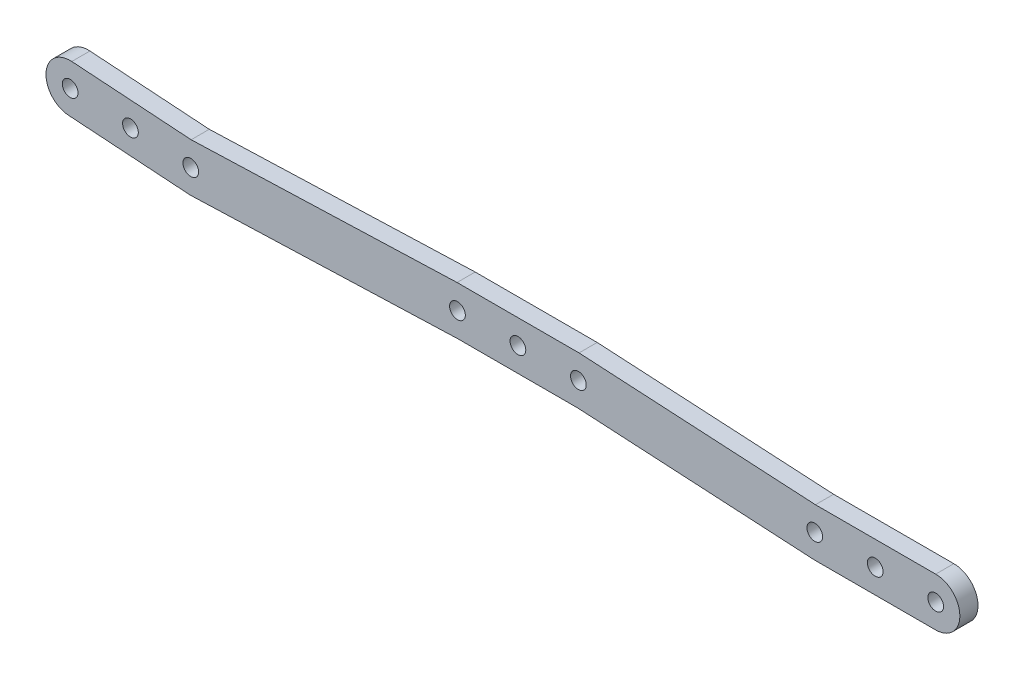
SolidWorks part; units mm, degrees
ref_plane "Front Plane" through (0, 0, 0) normal (0, 0, 1) x (1, 0, 0)
ref_plane "Top Plane" through (0, 0, 0) normal (0, 1, 0) x (1, 0, 0)
ref_plane "Right Plane" through (0, 0, 0) normal (1, 0, 0) x (0, 0, -1)
other "Configuration Table"
sketch "Sketch3" plane through (0, 0, 0) normal (0, 0, 1) x (1, 0, 0)
  line L8 (52.491, -11.9324) -> (42.491, -11.9324) construction
  line L9 (42.491, -11.9324) -> (32.491, -11.9324) construction
  line L10 (32.491, -11.9324) -> (-6.6156, -9.7382) construction
  line L11 (-6.6156, -9.7382) -> (-16.6156, -9.7382) construction
  line L12 (-16.6156, -9.7382) -> (-26.6156, -9.7382) construction
  line L13 (-26.6156, -9.7382) -> (-70.7349, -11.2865) construction
  line L14 (-70.7349, -11.2865) -> (-80.712, -10.61) construction
  line L15 (-80.712, -10.61) -> (-90.689, -9.9334) construction
  line L24 (52.491, -7.9324) -> (42.491, -7.9324)
  line L25 (42.491, -7.9324) -> (32.6031, -7.9324)
  line L26 (32.6031, -7.9324) -> (-6.5035, -5.7382)
  line L27 (-6.5035, -5.7382) -> (-16.6156, -5.7382)
  line L28 (-16.6156, -5.7382) -> (-26.6858, -5.7382)
  line L29 (-26.6858, -5.7382) -> (-70.6695, -7.2817)
  line L30 (-70.6695, -7.2817) -> (-80.4413, -6.6191)
  line L31 (-80.4413, -6.6191) -> (-90.4184, -5.9426)
  line L32 (52.491, -15.9324) -> (42.491, -15.9324)
  line L33 (42.491, -15.9324) -> (32.3788, -15.9324)
  line L34 (32.3788, -15.9324) -> (-6.7277, -13.7382)
  line L35 (-6.7277, -13.7382) -> (-16.6156, -13.7382)
  line L36 (-16.6156, -13.7382) -> (-26.5454, -13.7382)
  line L37 (-26.5454, -13.7382) -> (-70.8002, -15.2913)
  line L38 (-70.8002, -15.2913) -> (-80.9826, -14.6008)
  line L39 (-80.9826, -14.6008) -> (-90.9597, -13.9243)
  circle A21 centre (-90.689, -9.9334) radius 1.3
  circle A22 centre (-70.7349, -11.2865) radius 1.3
  circle A23 centre (-80.712, -10.61) radius 1.3
  circle A24 centre (-26.6156, -9.7382) radius 1.3
  circle A25 centre (-16.6156, -9.7382) radius 1.3
  circle A26 centre (-6.6156, -9.7382) radius 1.3
  circle A27 centre (32.491, -11.9324) radius 1.3
  circle A28 centre (42.491, -11.9324) radius 1.3
  circle A29 centre (52.491, -11.9324) radius 1.3
  arc A30 (-90.4184, -5.9426) -> (-90.9597, -13.9243) centre (-90.689, -9.9334) ccw
  arc A31 (52.491, -15.9324) -> (52.491, -7.9324) centre (52.491, -11.9324) ccw
  dimension "D3" = 4
extrude "Boss-Extrude4" add sketch "Sketch3" along normal blind 3
